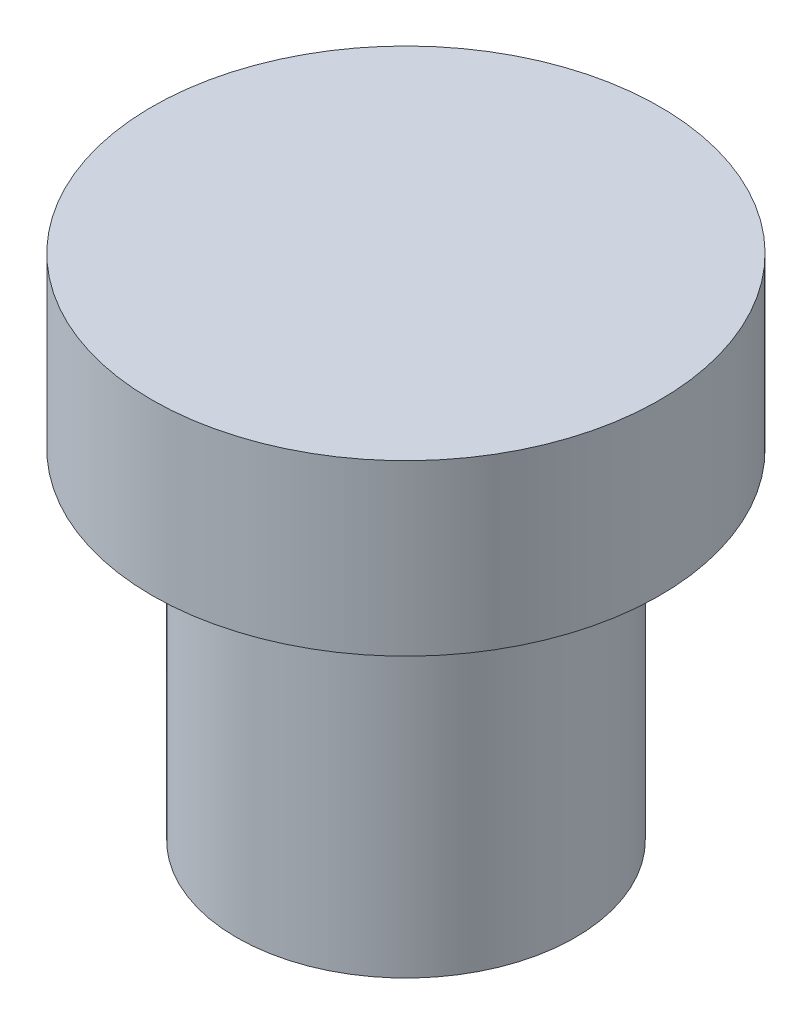
from build123d import *

# Parameters (mm, degrees)
SKETCH1_R           = 5
BOSS_EXTRUDE1_DEPTH = 10
SKETCH2_R           = 7.5
BOSS_EXTRUDE2_DEPTH = 5


with BuildPart() as part:
    # Sketch1 → Boss-Extrude1 (new body)
    with BuildSketch(Plane(origin=(0, 0, 0), x_dir=(1, 0, 0), z_dir=(0, 1, 0))):
        with Locations(Location((0, 0, 0), (0, 0, 270))):
            Circle(SKETCH1_R)
    extrude(amount=BOSS_EXTRUDE1_DEPTH)

    # Sketch2 → Boss-Extrude2 (add)
    with BuildSketch(Plane(origin=(0, 10, 0), x_dir=(1, 0, 0), z_dir=(0, 1, 0))):
        with Locations(Location((0, 0, 0), (0, 0, 270))):
            Circle(SKETCH2_R)
    extrude(amount=BOSS_EXTRUDE2_DEPTH)


solid = part.part
